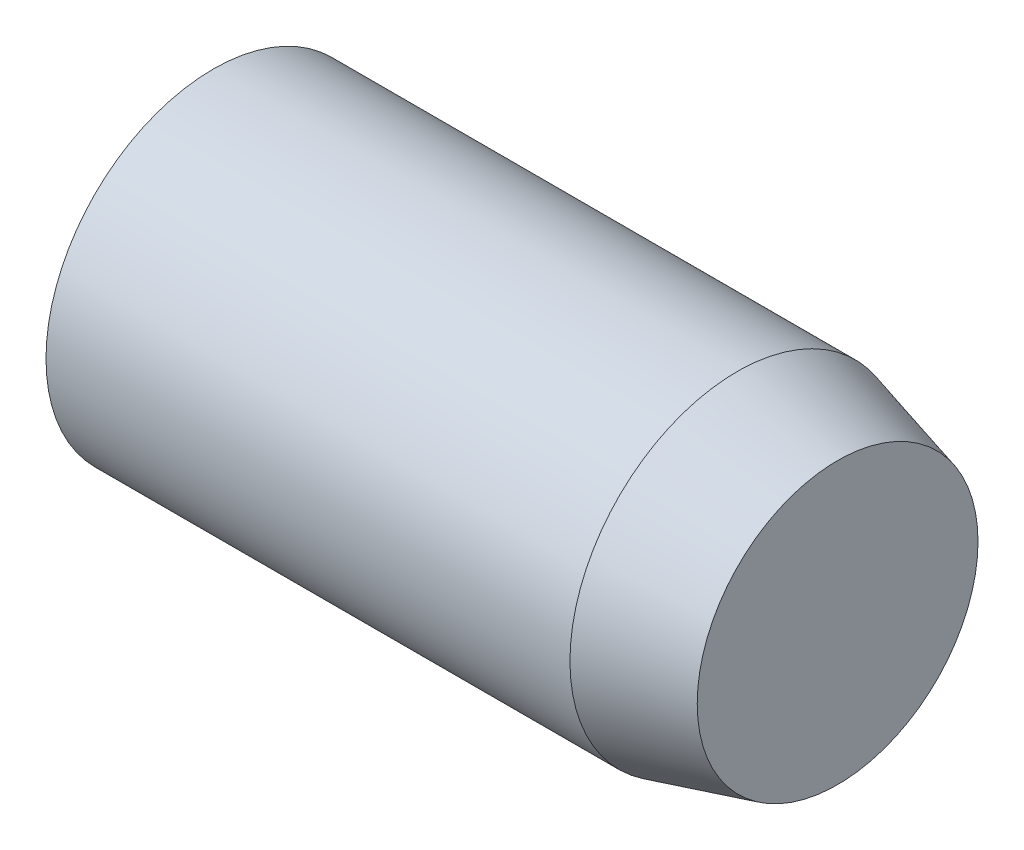
SolidWorks part; units mm, degrees
ref_plane "Front" through (0, 0, 0) normal (0, 0, 1) x (1, 0, 0)
ref_plane "Top" through (0, 0, 0) normal (0, 1, 0) x (1, 0, 0)
ref_plane "Right" through (0, 0, 0) normal (1, 0, 0) x (0, 0, -1)
sketch "Sketch1" plane through (0, 0, 0) normal (0, 1, 0) x (1, 0, 0)
  line L0 (-11.3907, 0) -> (1.7421, 0) construction
  line L1 (-1.5, -2.5) -> (0, -2.0981)
  line L2 (0, 0) -> (-10, 0)
  line L3 (0, 0) -> (0, -2.0981)
  line L4 (-1.5, -2.5) -> (-9.3301, -2.5)
  arc A0 (-10, 0) -> (-9.3301, -2.5) centre (-5, 0) ccw
  dimension "D2" = 10
  dimension "D1" = 5
  dimension "D3" = 1.5
  dimension "D4" = 15
  dimension "D5" = 10
revolve "Revolve1" add sketch "Sketch1" angle 360 mid plane about L0
